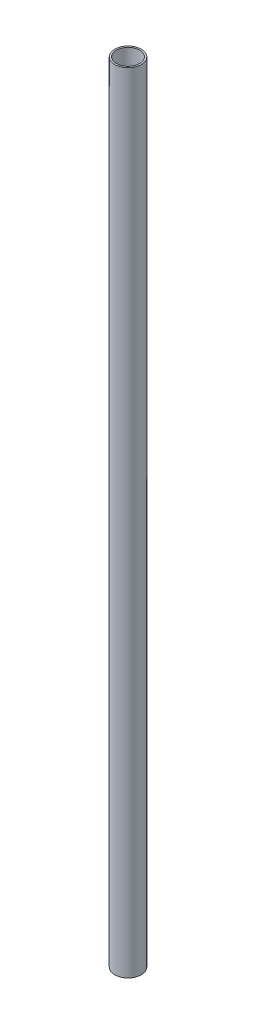
from build123d import *

# Parameters (mm, degrees)
SKETCH_1_R      = 8
SKETCH_1_R_2    = 7
EXTRUDE_1_DEPTH = 475


with BuildPart() as part:
    # 草图1 → 拉伸-薄壁1 (new body)
    with BuildSketch(Plane(origin=(0, 0, 0), x_dir=(1, 0, 0), z_dir=(0, 1, 0))):
        Circle(SKETCH_1_R)
        Circle(SKETCH_1_R_2, mode=Mode.SUBTRACT)
    extrude(amount=EXTRUDE_1_DEPTH)


solid = part.part
